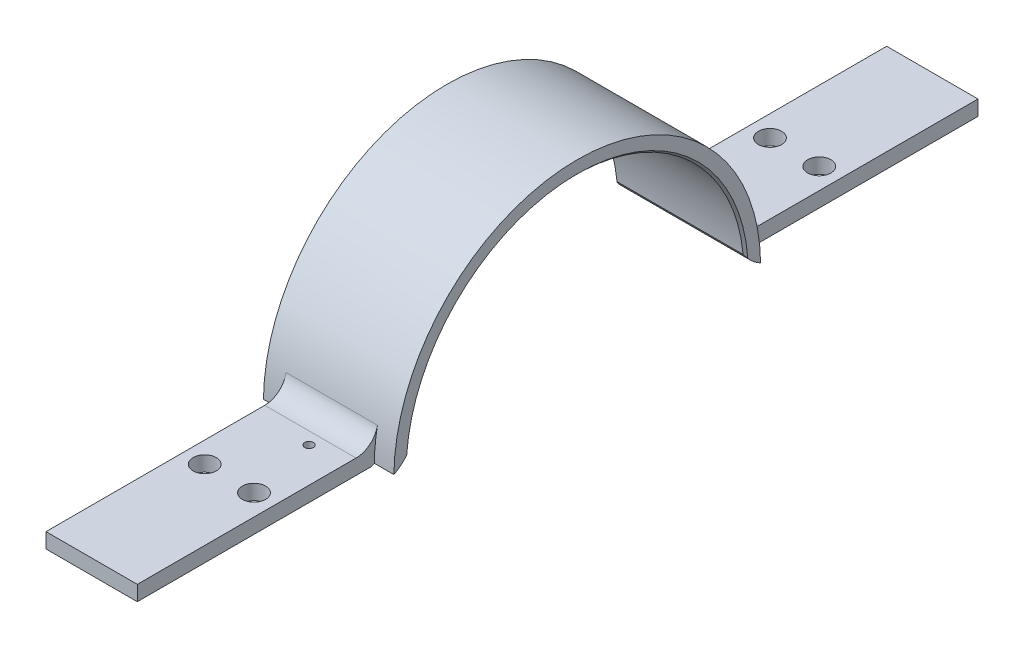
from build123d import *

# Parameters (mm, degrees)
BOSS_EXTRUDE1_DEPTH     = 90
FILLET1_R               = 30
FILLET2_R               = 55
CUT_EXTRUDE1_START      = -90
SKETCH2_R               = 233
CUT_EXTRUDE1_DEPTH      = 180
CUT_EXTRUDE2_DEPTH      = 640.147087923
CUT_EXTRUDE2_DEPTH_BACK = 640.147087923
SKETCH3_W               = 1220
SKETCH3_H               = 21.2
CUT_EXTRUDE3_DEPTH      = 27
MIRROR2_COPY_1_DEPTH    = 27
CUT_EXTRUDE4_DEPTH      = 640.147087923
CUT_EXTRUDE4_DEPTH_BACK = 640.147087923
SKETCH5_R               = 15
SKETCH5_R_2             = 6
CHAMFER1_SIZE           = 3
M36_TAPPED_HOLE1_D      = 32


with BuildPart() as part:
    # Sketch1 → Boss-Extrude1 (new, symmetric)
    with BuildSketch(Plane(origin=(0, 0, 0), x_dir=(0, 0, -1), z_dir=(1, 0, 0))):
        with BuildLine():
            Line((-580, 22), (-252.041663223, 22))
            ThreePointArc((-252.041663223, 22), (0, 253), (252.041663223, 22))
            Line((252.041663223, 22), (580, 22))
            Line((580, 22), (580, -3))
            Line((580, -3), (227.980262304, -3))
            ThreePointArc((227.980262304, -3), (0, 228), (-227.980262304, -3))
            Line((-227.980262304, -3), (-580, -3))
            Line((-580, -3), (-580, 22))
        make_face()
    extrude(amount=BOSS_EXTRUDE1_DEPTH, both=True)

    # Fillet1
    fillet1_edges = [part.edges().sort_by_distance(p)[0] for p in [
        (0, 22, 252.041663223),
        (0, 22, -252.041663223),
    ]]
    fillet(fillet1_edges, radius=FILLET1_R)

    # Fillet2
    fillet2_edges = [part.edges().sort_by_distance(p)[0] for p in [
        (0, -3, -227.980262304),
        (0, -3, 227.980262304),
    ]]
    fillet(fillet2_edges, radius=FILLET2_R)

    # Sketch2 → Cut-Extrude1 (cut)
    with BuildSketch(Plane(origin=(0, 0, 0), x_dir=(0, 0, -1), z_dir=(1, 0, 0)).offset(CUT_EXTRUDE1_START)):
        Circle(SKETCH2_R)
    extrude(amount=CUT_EXTRUDE1_DEPTH, mode=Mode.SUBTRACT)

    # Sketch3 → Cut-Extrude2 (cut, two sides: drawn at the far end of the back side and taken through both)
    with BuildSketch(Plane(origin=(0, 0, 0), x_dir=(0, 0, -1), z_dir=(1, 0, 0)).offset(-CUT_EXTRUDE2_DEPTH_BACK)):
        with Locations((0, -9.4)):
            Rectangle(SKETCH3_W, SKETCH3_H)
    extrude(amount=CUT_EXTRUDE2_DEPTH + CUT_EXTRUDE2_DEPTH_BACK, mode=Mode.SUBTRACT)

    # Sketch4 → Cut-Extrude3 (cut)
    with BuildSketch(Plane(origin=(90, 0, 0), x_dir=(0, 0, -1), z_dir=(1, 0, 0))):
        with BuildLine():
            Line((-598.01008044, 50), (-248.01008044, 50))
            ThreePointArc((-248.01008044, 50), (-252.546221213, 15.14615962), (-252.208247288, -20))
            Line((-252.208247288, -20), (-598.01008044, -20))
            Line((-598.01008044, -20), (-598.01008044, 50))
        make_face()
    cut_extrude3 = extrude(amount=-CUT_EXTRUDE3_DEPTH, mode=Mode.SUBTRACT)

    # Mirror1: Cut-Extrude3 across plane
    add(cut_extrude3.mirror(Plane.XY), mode=Mode.SUBTRACT)

    # Mirror2: Cut-Extrude3 across plane
    add(cut_extrude3.mirror(Plane(origin=(0, 0, 0), x_dir=(0, 0, 1), z_dir=(1, 0, 0))), mode=Mode.SUBTRACT)

    # Mirror2 copy 1 sketch → Mirror2 copy 1 (cut)
    with BuildSketch(Plane.ZY.offset(90)):
        with BuildLine():
            Line((-598.01008044, 50), (-248.01008044, 50))
            ThreePointArc((-248.01008044, 50), (-252.546221213, 15.14615962), (-252.208247288, -20))
            Line((-252.208247288, -20), (-598.01008044, -20))
            Line((-598.01008044, -20), (-598.01008044, 50))
        make_face()
    extrude(amount=-MIRROR2_COPY_1_DEPTH, mode=Mode.SUBTRACT)

    # Sketch5 → Cut-Extrude4 (cut, two sides: drawn at the far end of the back side and taken through both)
    with BuildSketch(Plane(origin=(0, 0, 0), x_dir=(1, 0, 0), z_dir=(0, 1, 0)).offset(-CUT_EXTRUDE4_DEPTH_BACK)):
        with Locations(Location((34, -390, 0), (0, 0, 90))):
            Circle(SKETCH5_R)
        with Locations(Location((34, 390, 0), (0, 0, 90))):
            Circle(SKETCH5_R)
        with Locations(Location((-34, -390, 0), (0, 0, 90))):
            Circle(SKETCH5_R)
        with Locations(Location((-34, 390, 0), (0, 0, 90))):
            Circle(SKETCH5_R)
        with Locations(Location((15, -295, 0), (0, 0, 90))):
            Circle(SKETCH5_R_2)
        with Locations(Location((-15, 295, 0), (0, 0, 90))):
            Circle(SKETCH5_R_2)
    extrude(amount=CUT_EXTRUDE4_DEPTH + CUT_EXTRUDE4_DEPTH_BACK, mode=Mode.SUBTRACT)

    # Chamfer1
    chamfer1_edges = [part.edges().sort_by_distance(p)[0] for p in [
        (-90, 233, 0),
        (90, 233, 0),
    ]]
    chamfer(chamfer1_edges, length=CHAMFER1_SIZE)

    # M36 Tapped Hole1 (through all)
    with Locations(Plane(origin=(0, 1.2, 0), x_dir=(-1, 0, 0), z_dir=(0, -1, 0))):
        with Locations((34, -390), (-34, -390), (-34, 390), (34, 390)):
            Hole(M36_TAPPED_HOLE1_D / 2)


solid = part.part
